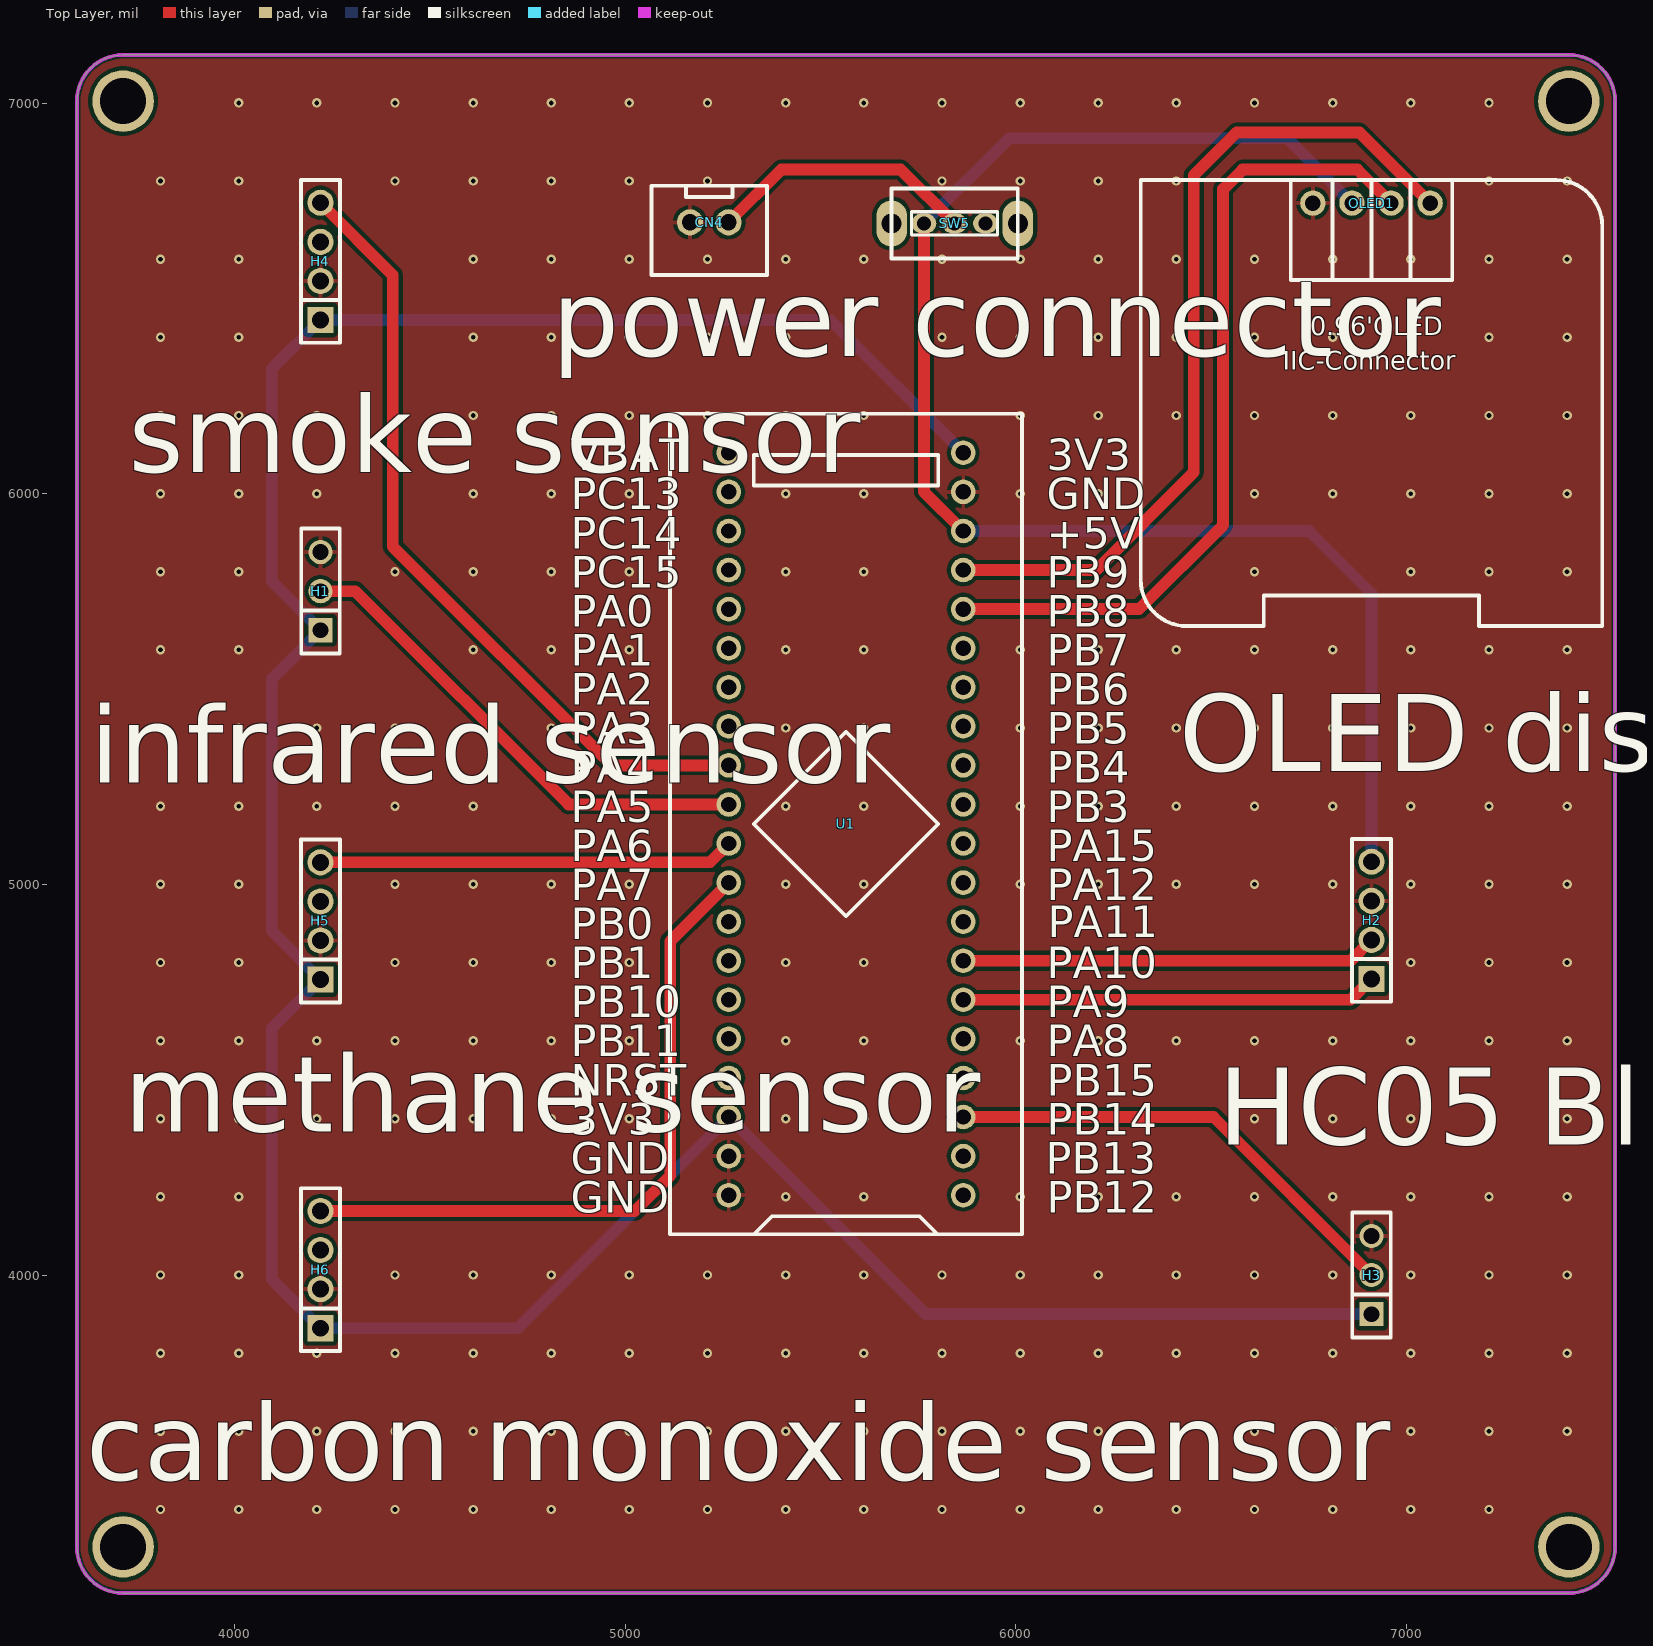
[diagram p0: Top Layer view]
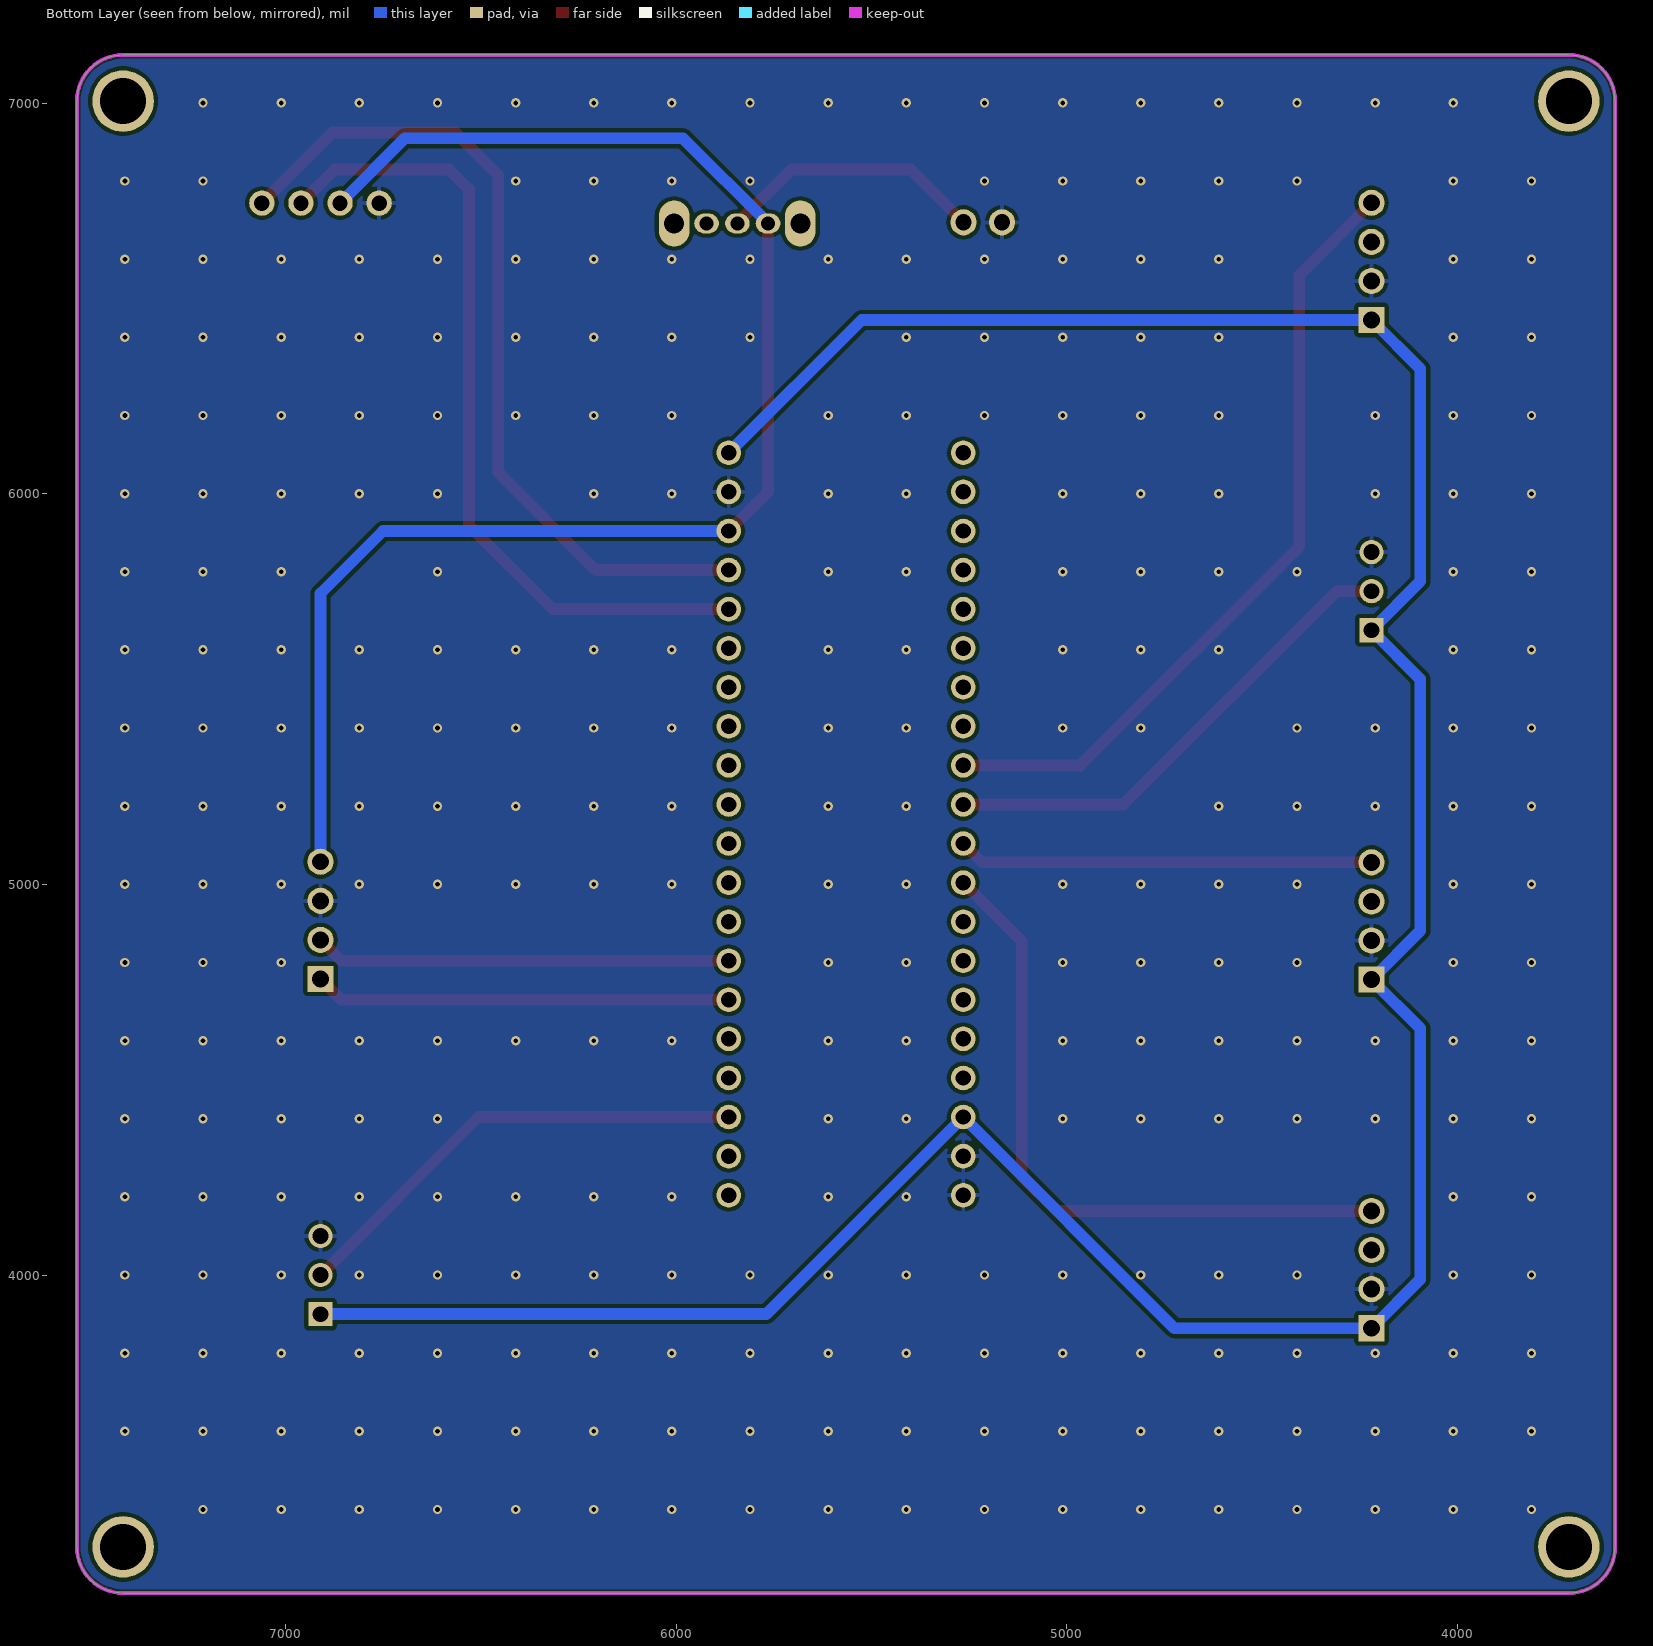
[diagram p1: Bottom Layer view, seen from below]
# Altium PCB MISC51056.pcbdoc
Units mil, origin at the board's own origin, x right, y up, seen from the top; angles counter-clockwise.
Board outline 3937.01 x 3937.01 mil, 2 copper layers (Top Layer, Bottom Layer), stack 62.206 mil thick; 10 components, 38 nets, 77 pads, 297 vias.

## Layer stack, top to bottom
Top Solder Mask Layer: solder mask 0.394, Dk 3.3
Top Layer: signal copper 1.379
Dielectric1: surface 59.449, FR4, Dk 4.5
Bottom Layer: signal copper 1.378
Bottom Solder Mask Layer: solder mask 0.394, Dk 3.3

## Board outline
3714.61,7123.5 ccw(c3714.61,7005.39) 3596.5,7005.39 3596.5,3304.61 ccw(c3714.61,3304.61) 3714.61,3186.5 7415.39,3186.5 ccw(c7415.39,3304.61) 7533.5,3304.61 7533.5,7005.39 ccw(c7415.39,7005.39) 7415.39,7123.5 3714.61,7123.5

## Design rules (kind name [scope] priority, off if disabled: settings)
BoardOutlineClearance copperThickness2oz_1 [All] p2 off: genericclearance=7.99 ignorepadtopadclearanceinfootprint=FALSE except(0: Arc-SplitContinuation Track-SplitContinuation SMDPad-SplitContinuation THPad-SplitContinuation Via-SplitContinuation Fill-SplitContinuation Region-SplitContinuation Poly-SplitContinuation Text-SplitContinuation Hole-SplitContinuation; 5.98: Arc-CutoutEdge Track-CutoutEdge SMDPad-CutoutEdge THPad-CutoutEdge Via-CutoutEdge Text-CutoutEdge; 6.9: Hole-OutlineEdge Hole-CutoutEdge; 10: Poly-OutlineEdge Poly-CutoutEdge; 11.81: Arc-OutlineEdge Track-OutlineEdge SMDPad-OutlineEdge THPad-OutlineEdge Via-OutlineEdge Fill-OutlineEdge Region-OutlineEdge Text-OutlineEdge Fill-CutoutEdge Region-CutoutEdge)
BoardOutlineClearance Plane_innerPlane_1 [All] p4 off: genericclearance=4.02 ignorepadtopadclearanceinfootprint=FALSE except(0: Arc-SplitContinuation Track-SplitContinuation SMDPad-SplitContinuation THPad-SplitContinuation Via-SplitContinuation Fill-SplitContinuation Region-SplitContinuation Poly-SplitContinuation Text-SplitContinuation Hole-SplitContinuation; 5.98: Arc-CutoutEdge Track-CutoutEdge SMDPad-CutoutEdge THPad-CutoutEdge Via-CutoutEdge Text-CutoutEdge; 6.9: Hole-OutlineEdge Hole-CutoutEdge; 10: Poly-OutlineEdge Poly-CutoutEdge; 11.81: Arc-OutlineEdge Track-OutlineEdge SMDPad-OutlineEdge THPad-OutlineEdge Via-OutlineEdge Fill-OutlineEdge Region-OutlineEdge Text-OutlineEdge Fill-CutoutEdge Region-CutoutEdge)
BoardOutlineClearance Copper_copperRegion_1 [All] p6 off: genericclearance=4.02 ignorepadtopadclearanceinfootprint=FALSE except(0: Arc-SplitContinuation Track-SplitContinuation SMDPad-SplitContinuation THPad-SplitContinuation Via-SplitContinuation Fill-SplitContinuation Region-SplitContinuation Poly-SplitContinuation Text-SplitContinuation Hole-SplitContinuation; 5.98: Arc-CutoutEdge Track-CutoutEdge SMDPad-CutoutEdge THPad-CutoutEdge Via-CutoutEdge Text-CutoutEdge; 6.9: Hole-OutlineEdge Hole-CutoutEdge; 10: Poly-OutlineEdge Poly-CutoutEdge; 11.81: Arc-OutlineEdge Track-OutlineEdge SMDPad-OutlineEdge THPad-OutlineEdge Via-OutlineEdge Fill-OutlineEdge Region-OutlineEdge Text-OutlineEdge Fill-CutoutEdge Region-CutoutEdge)
BoardOutlineClearance copperThickness1oz_1 [All] p8: genericclearance=4.02 ignorepadtopadclearanceinfootprint=FALSE except(0: Arc-SplitContinuation Track-SplitContinuation SMDPad-SplitContinuation THPad-SplitContinuation Via-SplitContinuation Fill-SplitContinuation Region-SplitContinuation Poly-SplitContinuation Text-SplitContinuation Hole-SplitContinuation; 5.98: Arc-CutoutEdge Track-CutoutEdge SMDPad-CutoutEdge THPad-CutoutEdge Via-CutoutEdge Text-CutoutEdge; 6.9: Hole-OutlineEdge Hole-CutoutEdge; 10: Poly-OutlineEdge Poly-CutoutEdge; 11.81: Arc-OutlineEdge Track-OutlineEdge SMDPad-OutlineEdge THPad-OutlineEdge Via-OutlineEdge Fill-OutlineEdge Region-OutlineEdge Text-OutlineEdge Fill-CutoutEdge Region-CutoutEdge)
Clearance copperThickness2oz [All] p1 off: gap=7.99 ignorepadtopadclearanceinfootprint=FALSE except(5.98: SMDPad-Track SMDPad-SMDPad THPad-Track SMDPad-THPad THPad-THPad Track-Via SMDPad-Via THPad-Via Via-Via Fill-SMDPad Region-SMDPad Fill-THPad Region-THPad Fill-Via Region-Via Fill-Fill Fill-Region Region-Region Arc-Track Arc-SMDPad Arc-THPad Arc-Via Fill-Arc Region-Arc Arc-Arc Text-Track SMDPad-Text Text-THPad Text-Via Fill-Text Region-Text Arc-Text Text-Text; 6.9: Hole-Track Hole-SMDPad Hole-THPad Hole-Via Fill-Hole Region-Hole Hole-Arc Hole-Text; 10: Poly-Track Poly-SMDPad Poly-THPad Poly-Via Poly-Fill Poly-Region Poly-Poly Poly-Arc Poly-Text Poly-Hole; 11.81: Fill-Track Region-Track)
Clearance Plane_innerPlane [All] p3 off: gap=4.02 ignorepadtopadclearanceinfootprint=FALSE except(5.98: SMDPad-Track SMDPad-SMDPad THPad-Track SMDPad-THPad THPad-THPad Track-Via SMDPad-Via THPad-Via Via-Via Fill-SMDPad Region-SMDPad Fill-THPad Region-THPad Fill-Via Region-Via Fill-Fill Fill-Region Region-Region Arc-Track Arc-SMDPad Arc-THPad Arc-Via Fill-Arc Region-Arc Arc-Arc Text-Track SMDPad-Text Text-THPad Text-Via Fill-Text Region-Text Arc-Text Text-Text; 6.9: Hole-Track Hole-SMDPad Hole-THPad Hole-Via Fill-Hole Region-Hole Hole-Arc Hole-Text; 10: Poly-Track Poly-SMDPad Poly-THPad Poly-Via Poly-Fill Poly-Region Poly-Poly Poly-Arc Poly-Text Poly-Hole; 11.81: Fill-Track Region-Track)
Clearance Copper_copperRegion [All] p5 off: gap=4.02 ignorepadtopadclearanceinfootprint=FALSE except(5.98: SMDPad-Track SMDPad-SMDPad THPad-Track SMDPad-THPad THPad-THPad Track-Via SMDPad-Via THPad-Via Via-Via Fill-SMDPad Region-SMDPad Fill-THPad Region-THPad Fill-Via Region-Via Fill-Fill Fill-Region Region-Region Arc-Track Arc-SMDPad Arc-THPad Arc-Via Fill-Arc Region-Arc Arc-Arc Text-Track SMDPad-Text Text-THPad Text-Via Fill-Text Region-Text Arc-Text Text-Text; 6.9: Hole-Track Hole-SMDPad Hole-THPad Hole-Via Fill-Hole Region-Hole Hole-Arc Hole-Text; 10: Poly-Track Poly-SMDPad Poly-THPad Poly-Via Poly-Fill Poly-Region Poly-Poly Poly-Arc Poly-Text Poly-Hole; 11.81: Fill-Track Region-Track)
Clearance copperThickness1oz [All] p7: gap=4.02 ignorepadtopadclearanceinfootprint=FALSE except(5.98: SMDPad-Track SMDPad-SMDPad THPad-Track SMDPad-THPad THPad-THPad Track-Via SMDPad-Via THPad-Via Via-Via Fill-SMDPad Region-SMDPad Fill-THPad Region-THPad Fill-Via Region-Via Fill-Fill Fill-Region Region-Region Arc-Track Arc-SMDPad Arc-THPad Arc-Via Fill-Arc Region-Arc Arc-Arc Text-Track SMDPad-Text Text-THPad Text-Via Fill-Text Region-Text Arc-Text Text-Text; 6.9: Hole-Track Hole-SMDPad Hole-THPad Hole-Via Fill-Hole Region-Hole Hole-Arc Hole-Text; 10: Poly-Track Poly-SMDPad Poly-THPad Poly-Via Poly-Fill Poly-Region Poly-Poly Poly-Arc Poly-Text Poly-Hole; 11.81: Fill-Track Region-Track)
DiffPairsRouting differentialPair [All] p1: maxlimit=6 minlimit=6 mostfreqgap=6 toplayer_minwidth=5 toplayer_prefwidth=10 toplayer_maxwidth=100 toplayer_mingap=6 toplayer_prefgap=6 toplayer_maxgap=6 bottomlayer_minwidth=5 bottomlayer_prefwidth=10 bottomlayer_maxwidth=100 bottomlayer_mingap=6 bottomlayer_prefgap=6 bottomlayer_maxgap=6 maxuncoupledlength=10
HoleToHoleClearance otherClearance [All] p1: gap=11.81 allowstackedmicrovias=TRUE
Length netLength [All] p1: minlimit=0 maxlimit=0
PasteMaskExpansion pasteMaskExpansion [All] p1: expansion=0
PlaneConnect innerPlane [All] p1: planeconnectstyle=Relief reliefexpansion=20 reliefentries=4 reliefconductorwidth=10 reliefairgap=10
PolygonConnect copperRegion [All] p1: connectstyle=Relief reliefconductorwidth=10 reliefentries=4 polygonreliefangle="90 Angle" airgapwidth=10 via.connectstyle=Relief via.reliefconductorwidth=10 via.reliefentries=4 via.polygonreliefangle="90 Angle" via.airgapwidth=10
RoutingVias viaSize [All] p1: holewidth=12.01 width=24.02 viastyle="Through Hole" minholewidth=11.81 minwidth=19.68 maxholewidth=248.03 maxwidth=393.7
SolderMaskExpansion solderMaskExpansion [IsVia] p1: expansion=-1000 istentingtop=TRUE
SolderMaskExpansion solderMaskExpansion [All] p2: expansion=2 istentingtop=FALSE
Width copperThickness2oz_2 [All] p1 off: maxlimit=100 minlimit=8 preferedwidth=10
Width copperThickness1oz_2 [All] p2: maxlimit=100 minlimit=5 preferedwidth=10

## Components (designator, comment, footprint, x,y, rotation, side; value= is the part's Value field where it differs from the comment)
CN4 "XH2.54*2P_through-hole" CONN-TH_2P-P2.50-XH2.54-2P 5215,6695 r0 top
H1 "" HDR-TH_3P-P2.54-V-F 4220,5750.96 r90 top
H2 "" HDR-TH_4P-P2.54-V-F 6910,4908.41 r90 top
H3 "" HDR-TH_3P-P2.54-V-F 6910,4000.59 r90 top
H4 "" HDR-TH_4P-P2.54-V-F 4220,6595 r90 top
H5 "" HDR-TH_4P-P2.54-V-F 4220,4906.91 r90 top
H6 "" HDR-TH_4P-P2.54-V-F 4220,4014.44 r90 top
OLED1 "" 0.96OLED_4P 6910,6744.11 r0 top
SW5 "" 拨动开关 5837.9,6692.05 r0 top
U1 "STM32F103C8T6-Card" CONN-TH_L53.3-W22.9_STM32F103C8T6-CARD 5565,5155 r90 top

## Footprints (in the part's own frame and the unit in brackets; to place one, negate y for a bottom-side part, rotate by r counter-clockwise, add the part's x,y. Pads: shape width x height; smd on the part's side, far side on the other; paste and mask are expansions set on the pad)
0.96OLED_4P [mm]
  round 1.65 hole 1 copper offset 0,0: 1(-3.81,-0.001) 2(-1.27,0.002) 3(1.27,0.002) 4(3.81,0.002)
  silkscreen extent -15,-27.5 15,1.5
CONN-TH_2P-P2.50-XH2.54-2P [mm]
  round 1.7 hole 1.05 paste+0 mask+0.05: 1(1.25,0) 2(-1.25,0)
  silkscreen extent -3.75,-3.42 3.75,2.37
CONN-TH_L53.3-W22.9_STM32F103C8T6-CARD [mm]
  round 1.6 hole 1: 1(-24.13,-7.62) 2(-21.59,-7.62) 3(-19.05,-7.62) 4(-16.51,-7.62) 5(-13.97,-7.62) 6(-11.43,-7.62) 7(-8.89,-7.62) 8(-6.35,-7.62) 9(-3.81,-7.62) 10(-1.27,-7.62) 11(1.27,-7.62) 12(3.81,-7.62) 13(6.35,-7.62) 14(8.89,-7.62) 15(11.43,-7.62) 16(13.97,-7.62) 17(16.51,-7.62) 18(19.05,-7.62) 19(21.59,-7.62) 20(24.13,-7.62) 21(24.13,7.62) 22(21.59,7.62) 23(19.05,7.62) 24(16.51,7.62) 25(13.97,7.62) 26(11.43,7.62) 27(8.89,7.62) 28(6.35,7.62) 29(3.81,7.62) 30(1.27,7.62) 31(-1.27,7.62) 32(-3.81,7.62) 33(-6.35,7.62) 34(-8.89,7.62) 35(-11.43,7.62) 36(-13.97,7.62) 37(-16.51,7.62) 38(-19.05,7.62) 39(-21.59,7.62) 40(-24.13,7.62)
  silkscreen extent -26.67,-11.43 26.67,11.43
HDR-TH_3P-P2.54-V-F [mil]
  rect 62x62 hole 40.16: 1(-100,0)
  round 62 hole 40.16: 2(0,0) 3(100,0)
  silkscreen extent -160,-49 160,49
HDR-TH_4P-P2.54-V-F [mm]
  rect 1.7x1.7 hole 1.1: 1(-3.81,0)
  round 1.7 hole 1.1: 2(-1.27,0) 3(1.27,0) 4(3.81,0)
  silkscreen extent -5.29,-1.27 5.29,1.27
拨动开关 [mil]
  oval 63x51.2 hole 35.4 paste+0 mask+2: 1(-73.4,0) 2(5,0) 3(84,0)
  oval 78.7x118.1 hole 51.2 paste+0 mask+2: 4(166.7,0) 5(-156.1,0)
  silkscreen extent -156,-90 167,90

## Free pads (board coordinates)
  round 157.48 hole 118.11: 1(3714.61,7005.39) 1(3714.61,3304.61) 1(7415.39,7005.39) 1(7415.39,3304.61)

## Via types
v1: diameter 24.02, hole 12, Top Layer to Bottom Layer, 297 vias

## Nets (pads, with @x,y where several pads share a name; then routed paths per layer and width w, separated by ;. In a path a pad name is that pad's centre, name@x,y a point inside that pad or via, vN(x,y) a via of type N, cw(c..) or ccw(c..) an arc to the next point about the centre after c; other vN are vias at no path point)
$1N17118: CN4.1 SW5.2 | length 691.7
  Top Layer w30: CN4.1 5399.22,6830 5704.95,6830 SW5.2
+5V: H2.4 OLED1.2 SW5.1 U1.18 | length 3881
  Top Layer w30: SW5.1 5764.5,6005.5 U1.18
  Bottom Layer w30: SW5.1 5982.45,6910 6694.16,6910 OLED1.2 ; U1.18 6750,5905 6910,5745 H2.4
GND: CN4.2 H1.3 H2.3 H3.3 H4.2 H5.2 H6.2 OLED1.1 U1.19 U1.39 U1.40
  other v1: 3810.6,3400.6 4010.6,3400.6 4210.6,3400.6 4410.6,3400.6 4610.6,3400.6 4810.6,3400.6 5010.6,3400.6 5210.6,3400.6 5410.6,3400.6 5610.6,3400.6 5810.6,3400.6 6010.6,3400.6 6210.6,3400.6 6410.6,3400.6 6610.6,3400.6 6810.6,3400.6 7010.6,3400.6 7210.6,3400.6 3810.6,3600.6 4010.6,3600.6 4210.6,3600.6 4410.6,3600.6 4610.6,3600.6 4810.6,3600.6 5010.6,3600.6 5210.6,3600.6 5410.6,3600.6 5610.6,3600.6 5810.6,3600.6 6010.6,3600.6 6210.6,3600.6 6410.6,3600.6 6610.6,3600.6 6810.6,3600.6 7010.6,3600.6 7210.6,3600.6 7410.6,3600.6 3810.6,3800.6 4010.6,3800.6 4210.6,3800.6 4410.6,3800.6 4610.6,3800.6 4810.6,3800.6 5010.6,3800.6 5210.6,3800.6 5410.6,3800.6 5610.6,3800.6 5810.6,3800.6 6010.6,3800.6 6210.6,3800.6 6410.6,3800.6 6610.6,3800.6 6810.6,3800.6 7010.6,3800.6 7210.6,3800.6 7410.6,3800.6 3810.6,4000.6 4010.6,4000.6 4410.6,4000.6 4610.6,4000.6 4810.6,4000.6 5010.6,4000.6 5210.6,4000.6 5410.6,4000.6 5610.6,4000.6 5810.6,4000.6 6010.6,4000.6 6210.6,4000.6 6410.6,4000.6 6610.6,4000.6 6810.6,4000.6 7010.6,4000.6 7210.6,4000.6 7410.6,4000.6 3810.6,4200.6 4010.6,4200.6 5410.6,4200.6 5610.6,4200.6 6010.6,4200.6 6210.6,4200.6 6410.6,4200.6 6610.6,4200.6 6810.6,4200.6 7010.6,4200.6 7210.6,4200.6 7410.6,4200.6 3810.6,4400.6 4010.6,4400.6 4210.6,4400.6 4410.6,4400.6 4610.6,4400.6 4810.6,4400.6 5010.6,4400.6 5410.6,4400.6 5610.6,4400.6 6610.6,4400.6 6810.6,4400.6 7010.6,4400.6 7210.6,4400.6 7410.6,4400.6 3810.6,4600.6 4010.6,4600.6 4210.6,4600.6 4410.6,4600.6 4610.6,4600.6 4810.6,4600.6 5010.6,4600.6 5410.6,4600.6 5610.6,4600.6 6010.6,4600.6 6210.6,4600.6 6410.6,4600.6 6610.6,4600.6 6810.6,4600.6 7010.6,4600.6 7210.6,4600.6 7410.6,4600.6 3810.6,4800.6 4010.6,4800.6 4410.6,4800.6 4610.6,4800.6 4810.6,4800.6 5010.6,4800.6 5410.6,4800.6 5610.6,4800.6 7010.6,4800.6 7210.6,4800.6 7410.6,4800.6 3810.6,5000.6 4010.6,5000.6 4410.6,5000.6 4610.6,5000.6 4810.6,5000.6 5010.6,5000.6 5410.6,5000.6 5610.6,5000.6 6010.6,5000.6 6210.6,5000.6 6410.6,5000.6 6610.6,5000.6 6810.6,5000.6 7010.6,5000.6 7210.6,5000.6 7410.6,5000.6 3810.6,5200.6 4010.6,5200.6 4210.6,5200.6 4410.6,5200.6 4610.6,5200.6 5410.6,5200.6 5610.6,5200.6 6010.6,5200.6 6210.6,5200.6 6410.6,5200.6 6610.6,5200.6 6810.6,5200.6 7010.6,5200.6 7210.6,5200.6 7410.6,5200.6 3810.6,5400.6 4010.6,5400.6 4210.6,5400.6 4410.6,5400.6 4810.6,5400.6 5010.6,5400.6 5410.6,5400.6 5610.6,5400.6 6010.6,5400.6 6210.6,5400.6 6410.6,5400.6 6610.6,5400.6 6810.6,5400.6 7010.6,5400.6 7210.6,5400.6 7410.6,5400.6 3810.6,5600.6 4010.6,5600.6 4610.6,5600.6 4810.6,5600.6 5010.6,5600.6 5410.6,5600.6 5610.6,5600.6 6010.6,5600.6 6210.6,5600.6 6410.6,5600.6 6610.6,5600.6 6810.6,5600.6 7010.6,5600.6 7210.6,5600.6 7410.6,5600.6 3810.6,5800.6 4010.6,5800.6 4410.6,5800.6 4610.6,5800.6 4810.6,5800.6 5010.6,5800.6 5410.6,5800.6 5610.6,5800.6 6610.6,5800.6 7010.6,5800.6 7210.6,5800.6 7410.6,5800.6 3810.6,6000.6 4010.6,6000.6 4210.6,6000.6 4610.6,6000.6 4810.6,6000.6 5010.6,6000.6 5410.6,6000.6 5610.6,6000.6 6010.6,6000.6 6210.6,6000.6 6610.6,6000.6 6810.6,6000.6 7010.6,6000.6 7210.6,6000.6 7410.6,6000.6 3810.6,6200.6 4010.6,6200.6 4210.6,6200.6 4610.6,6200.6 4810.6,6200.6 5010.6,6200.6 5210.6,6200.6 5410.6,6200.6 5610.6,6200.6 6010.6,6200.6 6210.6,6200.6 6410.6,6200.6 6610.6,6200.6 6810.6,6200.6 7010.6,6200.6 7210.6,6200.6 7410.6,6200.6 3810.6,6400.6 4010.6,6400.6 4610.6,6400.6 4810.6,6400.6 5010.6,6400.6 5210.6,6400.6 5410.6,6400.6 5810.6,6400.6 6010.6,6400.6 6210.6,6400.6 6410.6,6400.6 6610.6,6400.6 6810.6,6400.6 7010.6,6400.6 7210.6,6400.6 7410.6,6400.6 3810.6,6600.6 4010.6,6600.6 4610.6,6600.6 4810.6,6600.6 5010.6,6600.6 5210.6,6600.6 5410.6,6600.6 5610.6,6600.6 5810.6,6600.6 6010.6,6600.6 6210.6,6600.6 6410.6,6600.6 6610.6,6600.6 6810.6,6600.6 7010.6,6600.6 7210.6,6600.6 7410.6,6600.6 3810.6,6800.6 4010.6,6800.6 4410.6,6800.6 4610.6,6800.6 4810.6,6800.6 5010.6,6800.6 5210.6,6800.6 5810.6,6800.6 6010.6,6800.6 6210.6,6800.6 6410.6,6800.6 7210.6,6800.6 7410.6,6800.6 4010.6,7000.6 4210.6,7000.6 4410.6,7000.6 4610.6,7000.6 4810.6,7000.6 5010.6,7000.6 5210.6,7000.6 5410.6,7000.6 5610.6,7000.6 5810.6,7000.6 6010.6,7000.6 6210.6,7000.6 6410.6,7000.6 6610.6,7000.6 6810.6,7000.6 7010.6,7000.6 7210.6,7000.6
NRST: U1.37
PA0: U1.25
PA1: U1.26
PA2: U1.27
PA3: U1.28
PA4: H4.4 U1.29 | length 2048.6
  Top Layer w30: H4.4 4405,6560 4405,5865 4965,5305 U1.29
PA5: H1.2 U1.30 | length 1271.1
  Top Layer w30: H1.2 4309.04,5750.96 4855,5205 U1.30
PA6: H5.4 U1.31 | length 1064.9
  Top Layer w30: H5.4 5216.91,5056.91 U1.31
PA7: H6.4 U1.32 | length 1744.6
  Top Layer w30: H6.4 5024.44,4164.44 5115,4255 5115,4855 U1.32
PA8: U1.5
PA9: H2.1 U1.6 | length 1067.1
  Top Layer w30: U1.6 6856.58,4705 H2.1
PA10: H2.2 U1.7 | length 1067.1
  Top Layer w30: U1.7 6856.58,4805 H2.2
PA11: U1.8
PA12: U1.9
PA15: U1.10
PB0: U1.33
PB1: U1.34
PB3: U1.11
PB4: U1.12
PB5: U1.13
PB6: U1.14
PB7: U1.15
PB8: OLED1.3 U1.16 | length 2100.3
  Top Layer w30: U1.16 6315,5705 6530,5920 6530,6780 6580,6830 6874.16,6830 OLED1.3
PB9: OLED1.4 U1.17 | length 2179
  Top Layer w30: U1.17 6205,5805 6455,6055 6455,6815 6565,6925 6879.16,6925 OLED1.4
PB10: U1.35
PB11: U1.36
PB12: U1.1
PB13: U1.2
PB14: H3.2 U1.3 | length 1212.5
  Top Layer w30: U1.3 6505.58,4405 H3.2
PB15: U1.4
PC13: U1.22
PC14: U1.23
PC15: U1.24
VBAT: U1.21
VCC: H1.1 H3.1 H4.1 H5.1 H6.1 U1.20 U1.38 | length 7799.9
  Bottom Layer w30: U1.20 5525,6445 H4.1 4095,6320 4095,5775.96 H1.1 4095,5525.96 4095,4881.91 H5.1 4095,4631.91 4095,3989.44 H6.1 4724.44,3864.44 U1.38 5769.41,3900.59 H3.1
pads on no net: H4.3 H5.3 H6.3 SW5.3 SW5.4 SW5.5

## Polygon pours and split planes (outlines as drawn)
GND on Bottom Layer (solid, remove dead copper, pour order 2): 3525,7245 3525,3080 7700,3080 7700,7245
GND on Top Layer (solid, remove dead copper, pour order 2): 3000,7415 3000,3000 7930,3000 7930,7415

## Keep-outs
Board Outline Layer:
  the board outline again, w10

## Silkscreen, mask and mechanical layers (free items; w line width, h text height)
Top Silkscreen Layer:
  text "power connector" at 4812.87,6351.57 h196.85
  text "VBAT" at 4860.95,6060 h80
  text "3V3" at 6079.16,6060 h80
  text "smoke sensor" at 3728.77,6055.56 h196.85
  text "PC13" at 4860.95,5960 h80
  text "GND" at 6079.16,5960 h80
  text "PC14" at 4860.95,5860 h80
  text "+5V" at 6079.16,5860 h80
  text "PC15" at 4860.95,5760 h80
  text "PB9" at 6079.16,5760 h80
  text "PA0" at 4860.95,5660 h80
  text "PB8" at 6079.16,5660 h80
  text "PA1" at 4860.95,5560 h80
  text "PB7" at 6079.16,5560 h80
  text "PA2" at 4860.95,5460 h80
  text "PB6" at 6079.16,5460 h80
  text "PA3" at 4860.95,5360 h80
  text "PB5" at 6079.16,5360 h80
  text "OLED display" at 6418.02,5290.65 h196.85
  text "infrared sensor" at 3630.19,5259.94 h196.85
  text "PA4" at 4860.95,5260 h80
  text "PB4" at 6079.16,5260 h80
  text "PA5" at 4860.95,5160 h80
  text "PB3" at 6079.16,5160 h80
  text "PA6" at 4860.95,5060 h80
  text "PA15" at 6079.16,5060 h80
  text "PA7" at 4860.95,4960 h80
  text "PA12" at 6079.16,4960 h80
  text "PA11" at 6080.95,4865 h80
  text "PB0" at 4860.95,4860 h80
  text "PB1" at 4860.95,4760 h80
  text "PA10" at 6079.16,4760 h80
  text "PB10" at 4860.95,4660 h80
  text "PA9" at 6079.16,4660 h80
  text "PB11" at 4860.95,4560 h80
  text "PA8" at 6079.16,4560 h80
  text "NRST" at 4860.95,4460 h80
  text "PB15" at 6079.16,4460 h80
  text "methane sensor" at 3717.43,4367.47 h196.85
  text "3V3" at 4860.95,4360 h80
  text "PB14" at 6079.16,4360 h80
  text "HC05 Bluetooth" at 6517.49,4333.8 h196.85
  text "GND" at 4860.95,4260 h80
  text "PB13" at 6075.95,4260 h80
  text "GND" at 4860.95,4160 h80
  text "PB12" at 6079.16,4160 h80
  text "carbon monoxide sensor" at 3620,3475 h196.85
  text "DHT11 temperature/humidity" at 6368.66,3474.4 h196.85